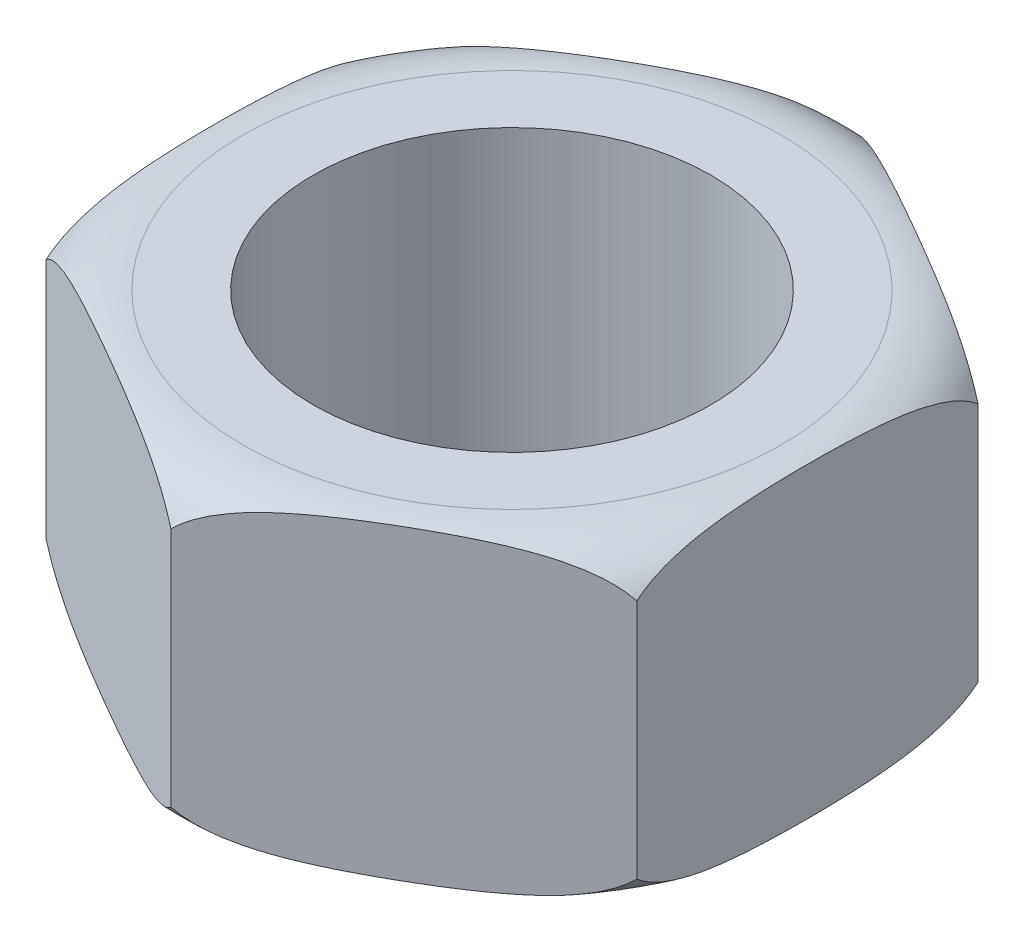
from build123d import *

# Parameters (mm, degrees)
SKETCH_1_R           = 16.5
BOSS_EXTRUDE_1_DEPTH = 13


with BuildPart() as part:
    # Sketch 1 → Boss-Extrude 1 (new, symmetric)
    with BuildSketch(Plane(origin=(0, 0, 0), x_dir=(1, 0, 0), z_dir=(0, 1, 0))):
        Polygon((0, 28.29016319), (-24.5, 14.145081595), (-24.5, -14.145081595), (0, -28.29016319), (24.5, -14.145081595), (24.5, 14.145081595), align=None)
        with Locations(Location((0, 0, 0), (0, 0, 90))):
            Circle(SKETCH_1_R, mode=Mode.SUBTRACT)
    extrude(amount=BOSS_EXTRUDE_1_DEPTH, both=True)

    # Sketch 2 → Cut-Revolve 1 (revolve, cut)
    with BuildSketch(Plane(origin=(0, 0, 0), x_dir=(0, 0, -1), z_dir=(1, 0, 0))):
        with BuildLine():
            Line((-22.29016319, 13), (-28.29016319, 13))
            Line((-28.29016319, 13), (-28.29016319, 10))
            add(Edge.make_bspline(
                [(-28.29016319, 10), (-27.028728561, 12.12896823), (-24.711520857, 13), (-22.29016319, 13)],
                knots=[0, 0, 0, 0, 1, 1, 1, 1], degree=3))
        make_face()
        with BuildLine():
            Line((-28.29016319, -13), (-28.29016319, -10))
            add(Edge.make_bspline(
                [(-28.29016319, -10), (-27.028728561, -12.12896823), (-24.711520857, -13), (-22.29016319, -13)],
                knots=[0, 0, 0, 0, 1, 1, 1, 1], degree=3))
            Line((-22.29016319, -13), (-28.29016319, -13))
        make_face()
    revolve(axis=Axis((0, 20.720193417, 0), (0, -1, 0)), mode=Mode.SUBTRACT)


solid = part.part
